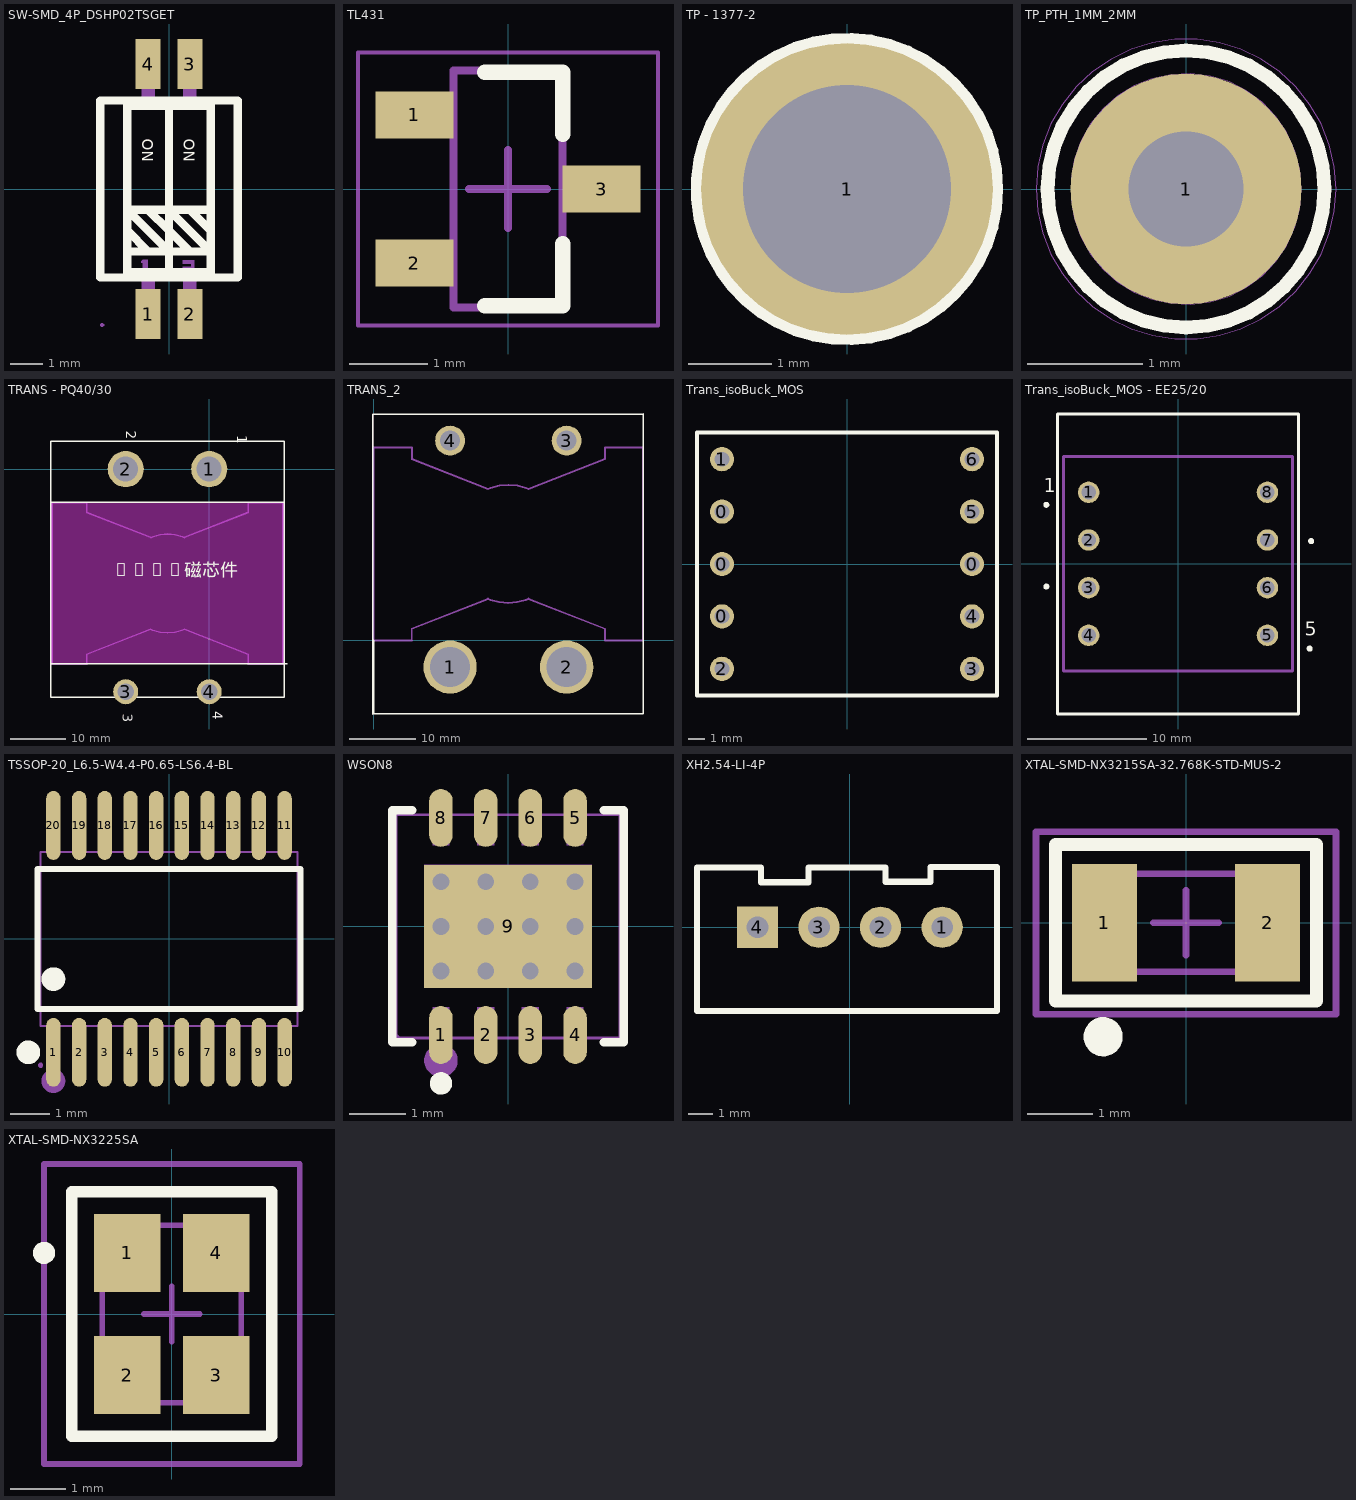
[diagram p0: the footprints below, top view; thin cyan lines are the x and y axes]
# Altium footprint library MISC82254-2.PcbLib: 93 footprints (part 6 of 6)
Each footprint in its own frame and in the unit in brackets; x right, y up, seen from the top. Pads: shape width x height; smd on the part's side, far side on the other; paste and mask are expansions set on the pad; w line width, h text height; cw(c..) or ccw(c..) is an arc to the next point about the centre after c.

## SW-SMD_4P_DSHP02TSGET [mil]
pads (4):
  rect 30x60 smd: 1(-25,-150) 2(25,-150) 3(25,150) 4(-25,150)
Top Overlay:
  lines w10: -50,-75 0,-75 ; -50,-50 -25,-75 ; -25,-25 0,-50 25,-75 ; 25,-25 50,-50 ; 50,-25 0,-25 ; 0,-100 -50,-100 -50,100 0,100 ; 0,-100 0,100 ; 0,-100 50,-100 50,100 0,100 ; 0,-100 0,100 ; 0,-75 50,-75 0,-25 ; 0,-75 -50,-25 0,-25 ; -82.68,-106.3 82.68,-106.3 82.68,106.3 -82.68,106.3 -82.68,-106.3
  text "ON" at 17.79,60.54 h12.98
  text "ON" at -32.21,60.54 h12.98
Mechanical 6:
  region: 20.67,-107.28 16.73,-107.28 16.73,-93.5 26.57,-93.5 26.57,-89.57 16.73,-89.57 16.73,-85.63 30.51,-85.63 30.51,-97.44 20.67,-97.44 20.67,-103.35 30.51,-103.35 30.51,-107.28
  region: -29.53,-84.65 -31.5,-84.65 -33.46,-86.61 -33.46,-88.58 -31.5,-88.58 -31.5,-106.3 -25.59,-106.3 -25.59,-84.65
Mechanical 15:
  region: -32.87,130.91 -32.87,164.37 -17.13,164.37 -17.13,130.91
  region: -32.87,105.91 -32.87,131.3 -17.13,131.3 -17.13,105.91
  region: -32.87,-164.37 -32.87,-130.91 -17.13,-130.91 -17.13,-164.37
  region: -32.87,-131.3 -32.87,-105.91 -17.13,-105.91 -17.13,-131.3
  region: 17.13,-164.37 17.13,-130.91 32.87,-130.91 32.87,-164.37
  region: 17.13,-131.3 17.13,-105.91 32.87,-105.91 32.87,-131.3
  region: 17.13,130.91 17.13,164.37 32.87,164.37 32.87,130.91
  region: 17.13,105.91 17.13,131.3 32.87,131.3 32.87,105.91
  region: -77.95,-163.19 -77.95,-162.21 -79.34,-160.83 -81.29,-160.83 -82.68,-162.21 -82.68,-163.19 -82.68,-164.17 -81.29,-165.55 -79.34,-165.55 -77.95,-164.17
  lines w2: -81.5,-106.3 81.5,-106.3 81.5,106.3 -81.5,106.3 -81.5,-106.3

## TL431 [mm] "SOT23, 3-Leads, Body 2.92x2.37mm, Pitch 0.95mm, IPC Medium Density"
height 1.12
pads (3):
  rect 1x0.6 smd: 1(-1.2,0.95) 2(-1.2,-0.95) 3(1.2,0)
Top Overlay:
  lines w0.2: -0.3,-1.5 0.7,-1.5 0.7,-0.7 ; -0.3,1.5 0.7,1.5 0.7,0.7
Mechanical 13:
  lines w0.1: -0.7,-1.52 -0.7,1.52 0.7,1.52 0.7,-1.52 -0.7,-1.52
Mechanical 15:
  lines w0.05: -1.925,-1.75 -1.925,1.75 1.925,1.75 1.925,-1.75 -1.925,-1.75
  lines w0.1: -0.5,0 0.5,0 ; 0,-0.5 0,0.5
3D body "SOT23-3N-TL431.step": height 1.12, standoff 0, extent -1.32,-1.52 1.32,1.52

## TP - 1377-2 [mm] "Keystone Micro Pin"
height 8
pads (1):
  round 3.5 hole 2.5: 1(0,0)
Top Overlay:
  circle w0.15: c0,0 r1.8
3D body: height 9, standoff 7, extent -0.999,-0.997 1,0.998
3D body: height 8, standoff -3, extent -1,-0.998 0.992,0.998
3D body: height 1, standoff 0, extent -1.608,-1.597 1.592,1.597

## TP_PTH_1MM_2MM [mm] "MCD-01506"
pads (1):
  round 2 hole 1 mask+0.05: 1(0,0)
Top Overlay:
  circle w0.12: c0,0 r1.2
Mechanical 14:
  circle w0.01: c0,0 r1
  text "'.Designator'" at -1.875,-0.4 h0.75
Mechanical 16:
  circle w0.01: c0,0 r1.3
3D body "5001.stp": height 4.94, standoff -2.68, extent -1.267,-1.27 1.267,1.26

## TRANS - PQ40/30 [mm]
pads (4):
  round 6.5 hole 4.5: 1(0,0) 2(-15,0)
  round 4.5 hole 3: 3(-15,-40) 4(0,-40)
Top Overlay:
  lines w0.254: -28.5,-6 13.5,-6 ; -28.45,-35 14.05,-35 ; -28.5,-41 13.5,-41 13.5,5 -28.5,5 -28.5,-41
  text "1" at 4.376,6.05 h3
  text "2" at -15.574,6.9 h3
  text "4" at -0.024,-43.55 h3
  text "3" at -16.174,-44 h3
  text "PQ40磁芯件" at -17.45,-20.036 h4
Keep-Out Layer:
  rectangle: -28.5,-35 13.5,-6
Mechanical 15:
  lines w0.3: -22.002,-33.341 -22.002,-35.041 -28.252,-35.041 -28.252,-6.041 -22.002,-6.041 ; -22.002,-33.266 -10.527,-28.801 -10.527,-28.774 -10.153,-28.949 -8.848,-29.298 -7.502,-29.416 -6.156,-29.298 -4.851,-28.949 -4.477,-28.774 -4.477,-28.801 6.998,-33.266 ; -22,-7.791 -10.525,-12.256 ; -22,-7.75 -22,-6.05 ; -10.5,-12.281 -10.5,-12.308 -10.126,-12.134 -8.821,-11.784 -7.475,-11.666 -6.129,-11.784 -4.824,-12.134 -4.45,-12.308 -4.45,-12.281 ; -4.475,-12.256 7,-7.791 ; 6.998,-33.341 6.998,-35.041 13.248,-35.041 13.248,-6.041 6.998,-6.041 ; 7,-7.75 7,-6.05

## TRANS_2 [mm]
pads (4):
  round 8 hole 6: 1(11.5,-4) 2(29,-4)
  round 4.5 hole 3: 3(29,30) 4(11.5,30)
Top Overlay:
  lines w0.254: -0.127,-11.049 -0.127,33.951 40.386,33.951 ; 0,0 0,-11 40.513,-11 40.513,34
Mechanical 13:
  lines w0.3: 5.74,0.009 5.74,1.709 ; 5.74,1.75 17.215,6.215 ; 5.742,27.225 17.217,22.76 17.217,22.733 17.591,22.908 18.896,23.257 20.242,23.375 21.588,23.257 22.893,22.908 23.267,22.733 23.267,22.76 34.742,27.225 ; 5.742,27.3 5.742,29 ; 5.75,0 0,0 0,29 5.75,29 ; 17.19,6.24 17.19,6.267 17.564,6.092 18.869,5.743 20.215,5.625 21.561,5.743 22.866,6.092 23.24,6.267 23.24,6.24 ; 23.265,6.215 34.74,1.75 ; 34.74,0.009 34.74,1.709 ; 34.742,0 40.492,0 ; 34.742,27.3 34.742,29 ; 34.744,28.991 40.494,28.991 40.494,-0.009
  text "PQ40磁芯" at 14.859,13.014 h3

## Trans_isoBuck_MOS [mm]
height 2.8
pads (10):
  round 1.5 hole 0.9: 0(-7.75,-3.25) 0(-7.75,0) 0(-7.75,3.25) 0(7.75,0) 1(-7.75,6.5) 2(-7.75,-6.5) 3(7.75,-6.5) 4(7.75,-3.25) 5(7.75,3.25) 6(7.75,6.5)
Top Overlay:
  lines w0.254: -9.3,-8.15 9.3,-8.15 9.3,8.15 -9.3,8.15 -9.3,-8.15

## Trans_isoBuck_MOS - EE25/20 [mm]
height 2.8
pads (8):
  round 1.8 hole 1.2: 1(-7.5,6) 2(-7.5,2) 3(-7.5,-2) 4(-7.5,-6) 5(7.5,-6) 6(7.5,-2) 7(7.5,2) 8(7.5,6)
Top Overlay:
  circle w0.254: c11.176,1.905 r0.127
  circle w0.254: c11.049,-7.112 r0.127
  circle w0.254: c-11.049,-1.905 r0.127
  circle w0.254: c-11.049,4.953 r0.127
  lines w0.254: -10.1,-12.6 -10.1,12.573 10.1,12.573 10.1,-12.6 -10.1,-12.6
  text "5" at 10.625,-6.456 h2
  text "1" at -11.285,5.588 h2
Mechanical 13:
  lines w0.254: -9.6,-9 -9.6,9 9.6,9 9.6,-9 -9.6,-9
3D body: height 16, standoff 0, extent -10.033,-12.573 10.16,12.573

## TSSOP-20_L6.5-W4.4-P0.65-LS6.4-BL [mm]
pads (20):
  oval 0.364x1.742 smd: 1(-2.925,-2.871) 2(-2.275,-2.871) 3(-1.625,-2.871) 4(-0.975,-2.871) 5(-0.325,-2.871) 6(0.325,-2.871) 7(0.975,-2.871) 8(1.625,-2.871) 9(2.275,-2.871) 10(2.925,-2.871) 11(2.925,2.871) 12(2.275,2.871) 13(1.625,2.871) 14(0.975,2.871) 15(0.325,2.871) 16(-0.325,2.871) 17(-0.975,2.871) 18(-1.625,2.871) 19(-2.275,2.871) 20(-2.925,2.871)
Top Overlay:
  circle w0.3: c-3.559,-2.871 r0.15
  circle w0.3: c-2.925,-1.019 r0.15
  lines w0.152: -3.326,-1.771 3.326,-1.771 3.326,1.771 -3.326,1.771 -3.326,-1.771
Mechanical 6:
  circle w0.3: c-2.925,-3.6 r0.15
Mechanical 15:
  drawing of 45 lines, arcs and shapes, not listed
3D body "SN74ACT244PWR.stp": height 1.13, standoff 0, extent -3.25,-3.2 3.25,3.2

## WSON8 [mm]
pads (9):
  oval 0.42x1.035 smd: 1(-1.2,-1.943) 2(-0.4,-1.943) 3(0.4,-1.943) 4(1.2,-1.943) 5(1.2,1.943) 6(0.4,1.943) 7(-0.4,1.943) 8(-1.2,1.943)
  rect 3x2.2 smd: 9(0,0)
via 1.2,-0.8 diameter 0.5 hole 0.3
via 0.4,-0.8 diameter 0.5 hole 0.3
via -0.4,-0.8 diameter 0.5 hole 0.3
via -1.2,-0.8 diameter 0.5 hole 0.3
via -1.2,0 diameter 0.5 hole 0.3
via -0.4,0 diameter 0.5 hole 0.3
via 0.4,0 diameter 0.5 hole 0.3
via 1.2,0 diameter 0.5 hole 0.3
via 1.2,0.8 diameter 0.5 hole 0.3
via 0.4,0.8 diameter 0.5 hole 0.3
via -0.4,0.8 diameter 0.5 hole 0.3
via -1.2,0.8 diameter 0.5 hole 0.3
Top Overlay:
  circle w0.2: c-1.2,-2.81 r0.1
  lines w0.152: -1.715,-2.076 -2.076,-2.076 -2.076,2.076 -1.715,2.076 ; 1.715,-2.076 2.076,-2.076 2.076,2.076 1.715,2.076
Mechanical 6:
  circle w0.3: c-1.2,-2.4 r0.15
Mechanical 15:
  region: -1.94,-2 -1.94,-1.975 -1.975,-1.94 -2.025,-1.94 -2.06,-1.975 -2.06,-2 -2.06,-2.025 -2.025,-2.06 -1.975,-2.06 -1.94,-2.025
  region: -1.5,1.1 1.5,1.1 1.5,-1.1 -1.5,-1.1
  region: 1.05,1.95 1.05,1.45 1.35,1.45 1.35,1.95
  region: 0.25,1.95 0.25,1.45 0.55,1.45 0.55,1.95
  region: -0.55,1.95 -0.55,1.45 -0.25,1.45 -0.25,1.95
  region: -1.35,1.95 -1.35,1.45 -1.05,1.45 -1.05,1.95
  region: 1.05,-1.95 1.05,-1.45 1.35,-1.45 1.35,-1.95
  region: 0.25,-1.95 0.25,-1.45 0.55,-1.45 0.55,-1.95
  region: -0.55,-1.95 -0.55,-1.45 -0.25,-1.45 -0.25,-1.95
  region: -1.35,-1.95 -1.35,-1.45 -1.05,-1.45 -1.05,-1.95
  lines w0.051: -2,-2 2,-2 2,2 -2,2 -2,-2
3D body "LM34927SD_NOPB.stp": height 0.8, standoff 0, extent -2,-2 2,2

## XH2.54-LI-4P [mm] "接插件，4P"
pads (4):
  round 1.7 hole 0.9: 1(3.81,0) 2(1.27,0) 3(-1.27,0)
  rect 1.7x1.7 hole 0.9: 4(-3.81,0)
Top Overlay:
  lines w0.254: -6.299,-3.454 -6.299,2.464 -3.658,2.464 -3.658,1.854 -1.702,1.854 -1.702,2.464 1.473,2.464 1.473,1.88 3.327,1.88 3.327,2.489 6.071,2.489 6.071,-3.454 -6.299,-3.454
3D body "XH2.54-4P.STEP": height 7.03, standoff -2.47, extent -6.31,-3.3 6.31,2.4

## XTAL-SMD-NX3215SA-32.768K-STD-MUS-2 [mm] "Crystal; 3.2mm W X 1.5mm L X 0.9mm H body"
height 0.9
pads (2):
  rect 1x1.8 smd paste+0 mask+0: 1(-1.25,0) 2(1.25,0)
Top Overlay:
  circle w0.3: c-1.27,-1.746 r0.15
  lines w0.2: -2,-1.2 2,-1.2 2,1.2 -2,1.2 -2,-1.2
Mechanical 3:
  text ".DESIGNATOR" at -0.263,-2.419 h1.2
Mechanical 13:
  lines w0.1: -1.6,-0.75 -1.6,0.75 1.6,0.75 1.6,-0.75 -1.6,-0.75
Mechanical 15:
  lines w0.1: -0.5,0 0.5,0 ; 0,-0.5 0,0.5 ; -2.3,-1.4 -2.3,1.4 2.3,1.4 2.3,-1.4 -2.3,-1.4
3D body: height 0.9, standoff 0.9, extent -1.409,0.28 -1.11,0.58
3D body: height 0.9, standoff 0, extent -1.6,-0.75 1.6,0.75

## XTAL-SMD-NX3225SA [mm] "Crystal; 3.2mm W X 2.5mm L X 0.6mm H body"
height 0.6
pads (4):
  rect 1.2x1.4 smd paste+0 mask+0: 1(-0.8,1.1) 2(-0.8,-1.1) 3(0.8,-1.1) 4(0.8,1.1)
Top Overlay:
  circle w0.2: c-2.3,1.1 r0.1
  lines w0.2: -1.8,-2.2 1.8,-2.2 1.8,2.2 -1.8,2.2 -1.8,-2.2
Mechanical 3:
  text ".DESIGNATOR" at -2.16,-3.434 h1.2
Mechanical 13:
  lines w0.1: -1.25,-1.6 -1.25,1.6 1.25,1.6 1.25,-1.6 -1.25,-1.6
Mechanical 15:
  lines w0.1: -0.5,0 0.5,0 ; 0,-0.5 0,0.5 ; -2.3,-2.7 2.3,-2.7 2.3,2.7 -2.3,2.7 -2.3,-2.7
3D body: height 0.35, standoff 0.05, extent -1.25,-1.6 1.25,1.6
3D body: height 0.05, standoff 0, extent 0.35,0.6 1.25,1.6
3D body: height 0.05, standoff 0, extent 0.35,-1.6 1.25,-0.6
3D body: height 0.05, standoff 0, extent -1.25,-1.6 -0.35,-0.6
3D body: height 0.05, standoff 0, extent -1.25,0.6 -0.35,1.6
3D body: height 0.48, standoff 0.25, extent -1.2,-1.53 1.2,1.53
3D body: height 0.6, standoff 0.25, extent -1.05,-1.375 1.05,1.375